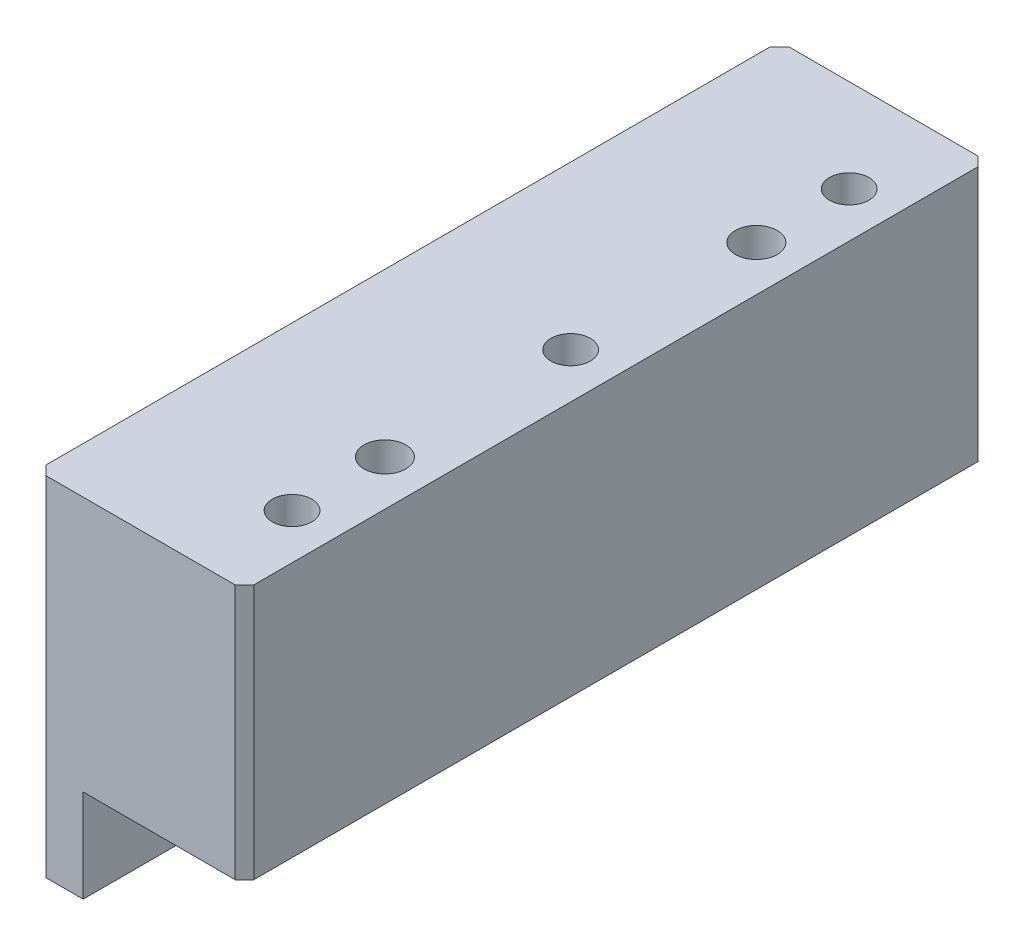
from build123d import *

# Parameters (mm, degrees)
SKETCH1_W                                           = 44.75
SKETCH1_H                                           = 160
BOSS_EXTRUDE1_DEPTH                                 = 75
SKETCH5_W                                           = 34.75
SKETCH5_H                                           = 160
CUT_EXTRUDE3_DEPTH                                  = 20
F_8_5_8_5_DIAMETER_HOLE1_D                          = 8.5
CHAMFER2_SIZE                                       = 2
CBORE_FOR_M8_HEX_SOCKET_HEAD_CAP_SCREW1_D           = 9
CBORE_FOR_M8_HEX_SOCKET_HEAD_CAP_SCREW1_CBORE_D     = 15
CBORE_FOR_M8_HEX_SOCKET_HEAD_CAP_SCREW1_CBORE_DEPTH = 40


with BuildPart() as part:
    # Sketch1 → Boss-Extrude1 (new body)
    with BuildSketch(Plane(origin=(0, 0, 0), x_dir=(1, 0, 0), z_dir=(0, 1, 0))):
        Rectangle(SKETCH1_W, SKETCH1_H)
    extrude(amount=BOSS_EXTRUDE1_DEPTH)

    # Sketch5 → Cut-Extrude3 (cut)
    with BuildSketch(Plane.XZ):
        with Locations((5, 0)):
            Rectangle(SKETCH5_W, SKETCH5_H)
    extrude(amount=-CUT_EXTRUDE3_DEPTH, mode=Mode.SUBTRACT)

    # Ø8.5 (8.5) Diameter Hole1 (through all)
    with Locations(Plane(origin=(0, 75, 0), x_dir=(-1, 0, 0), z_dir=(0, 1, 0))):
        with Locations((-12.625, -60), (-12.625, 0), (-12.625, 60)):
            Hole(F_8_5_8_5_DIAMETER_HOLE1_D / 2)

    # Chamfer2
    chamfer2_edges = [part.edges().sort_by_distance(p)[0] for p in [
        (22.375, 47.5, 80),
        (-22.375, 37.5, 80),
        (-22.375, 37.5, -80),
        (22.375, 47.5, -80),
    ]]
    chamfer(chamfer2_edges, length=CHAMFER2_SIZE)

    # CBORE for M8 Hex Socket Head Cap Screw1 (through all)
    with Locations(Plane.XZ.offset(-20)):
        with Locations((12.625, 40), (12.625, -40)):
            CounterBoreHole(CBORE_FOR_M8_HEX_SOCKET_HEAD_CAP_SCREW1_D / 2, CBORE_FOR_M8_HEX_SOCKET_HEAD_CAP_SCREW1_CBORE_D / 2, CBORE_FOR_M8_HEX_SOCKET_HEAD_CAP_SCREW1_CBORE_DEPTH)


solid = part.part
